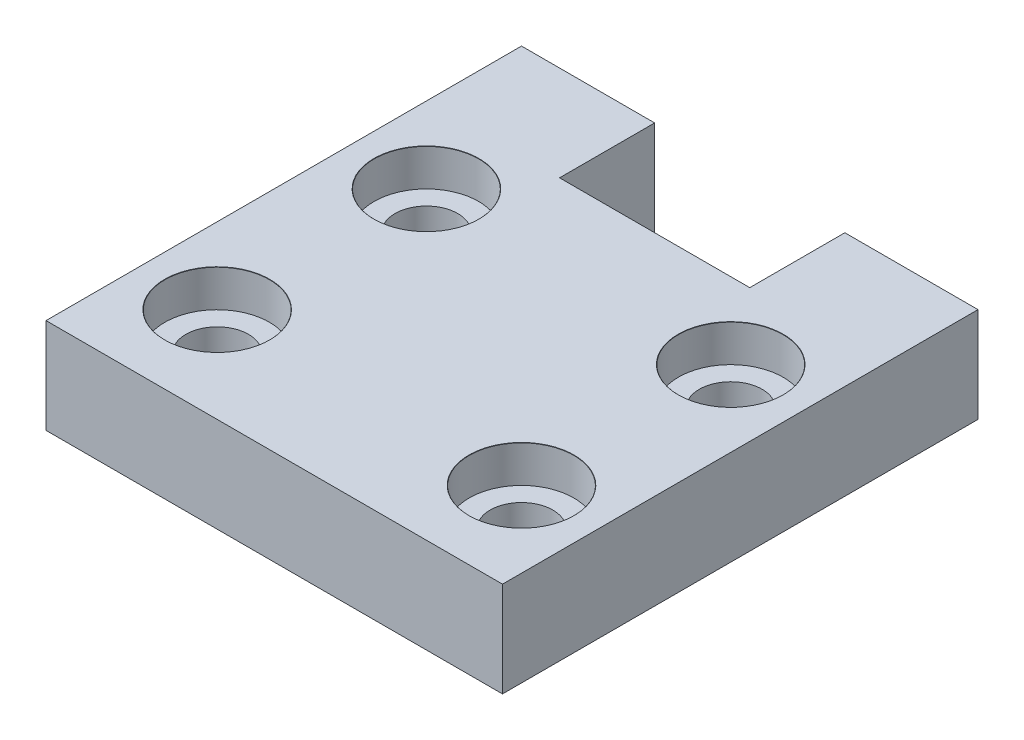
SolidWorks part; units mm, degrees
ref_plane "Front Plane" through (0, 0, 0) normal (0, 0, 1) x (1, 0, 0)
ref_plane "Top Plane" through (0, 0, 0) normal (0, 1, 0) x (1, 0, 0)
ref_plane "Right Plane" through (0, 0, 0) normal (1, 0, 0) x (0, 0, -1)
sketch "Sketch1" plane through (0, 0, 0) normal (0, 1, 0) x (1, 0, 0)
  line L1 (-24, 25) -> (24, 25)
  line L2 (-24, 25) -> (-24, -25)
  line L3 (-24, -25) -> (24, -25)
  line L4 (24, 25) -> (24, -25)
  line L5 (-24, 25) -> (24, -25) construction
  line L6 (-24, -25) -> (24, 25) construction
  point P0 (0, 0)
  dimension "D1" = 48
  dimension "D2" = 50
extrude "Boss-Extrude1" add sketch "Sketch1" along normal blind 10
sketch "Sketch2" plane through (0, 10, 0) normal (0, 1, 0) x (1, 0, 0)
  line L0 (24, 25) -> (-24, 25) construction
  line L1 (-10, 35) -> (10, 35)
  line L2 (-10, 35) -> (-10, 15)
  line L3 (-10, 15) -> (10, 15)
  line L4 (10, 35) -> (10, 15)
  line L5 (-10, 35) -> (10, 15) construction
  line L6 (-10, 15) -> (10, 35) construction
  point P0 (0, 25)
  dimension "D1" = 20
  dimension "D2" = 20
extrude "Cut-Extrude1" cut sketch "Sketch2" against normal blind 10
hole_wizard "CBORE for M6 Cheese Head Screw1" positions "Sketch3" profile "Sketch4" counterbore size "M6" standard "ISO"
sketch "Sketch3" plane through (0, 10, 0) normal (0, 1, 0) x (1, 0, 0)
  line L0 (0, 15) -> (0, -25) construction
  line L1 (-10, 15) -> (10, 15) construction
  line L2 (-24, -25) -> (24, -25) construction
  line L8 (-16, -15) -> (-16, 7) construction
  line L9 (-16, 7) -> (16, 7) construction
  line L10 (16, 7) -> (16, -15) construction
  line L11 (16, -15) -> (-16, -15) construction
  line L13 (-10, 25) -> (-24, 25) construction
  line L14 (-16, -4) -> (16, -4) construction
  point P0 (-16, 7)
  point P2 (-16, -15)
  point P4 (16, -15)
  point P6 (16, 7)
  point P31 (0, 7)
  dimension "D1" = 22
  dimension "D2" = 10
  dimension "D3" = 18
  dimension "D4" = 10
  dimension "D5" = 32
sketch "Sketch4" plane through (-16, 10, -7) normal (1, 0, 0) x (0, 0, 1)
  line L0 (0, 0) -> (0, 11.9828)
  line L1 (0, 11.9828) -> (3.3, 10)
  line L2 (3.3, 10) -> (3.3, 3.9)
  line L3 (3.3, 3.9) -> (5.5, 3.9)
  line L5 (5.5, 3.9) -> (5.5, 0.025)
  line L6 (5.5, 0.025) -> (5.525, 0)
  line L7 (5.525, 0) -> (0, 0)
  line L8 (-5.5, 0.025) -> (-5.525, 0) construction
  line L10 (0, 11.9828) -> (-3.3, 10) construction
  line L11 (0, -6.35) -> (0, 107.95) construction
  dimension "Hole Dia." = 6.6
  dimension "Hole Depth" = 10
  dimension "C'Bore Dia." = 11
  dimension "C'Bore Depth" = 3.9
  dimension "Near C'Sink Dia." = 11.05
  dimension "Near C'Sink Angle" = 90
  dimension "Drill Angle" = 118
